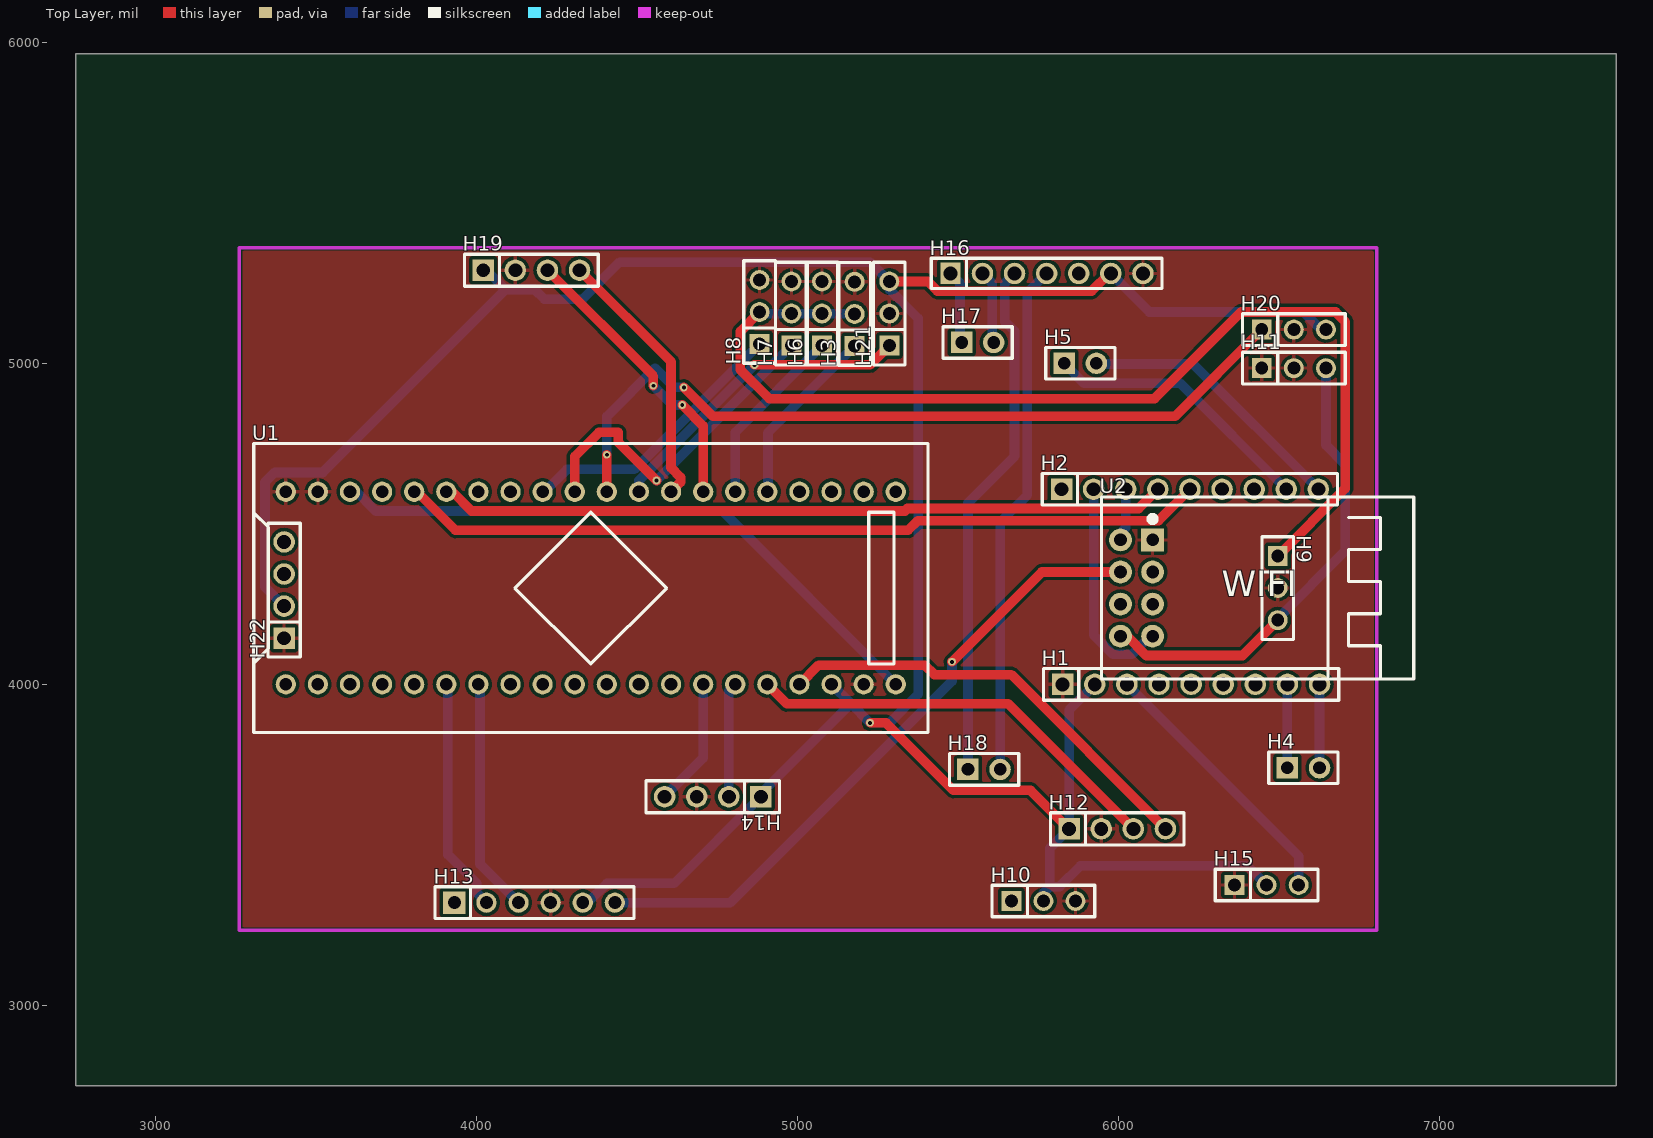
[diagram p0: Top Layer view]
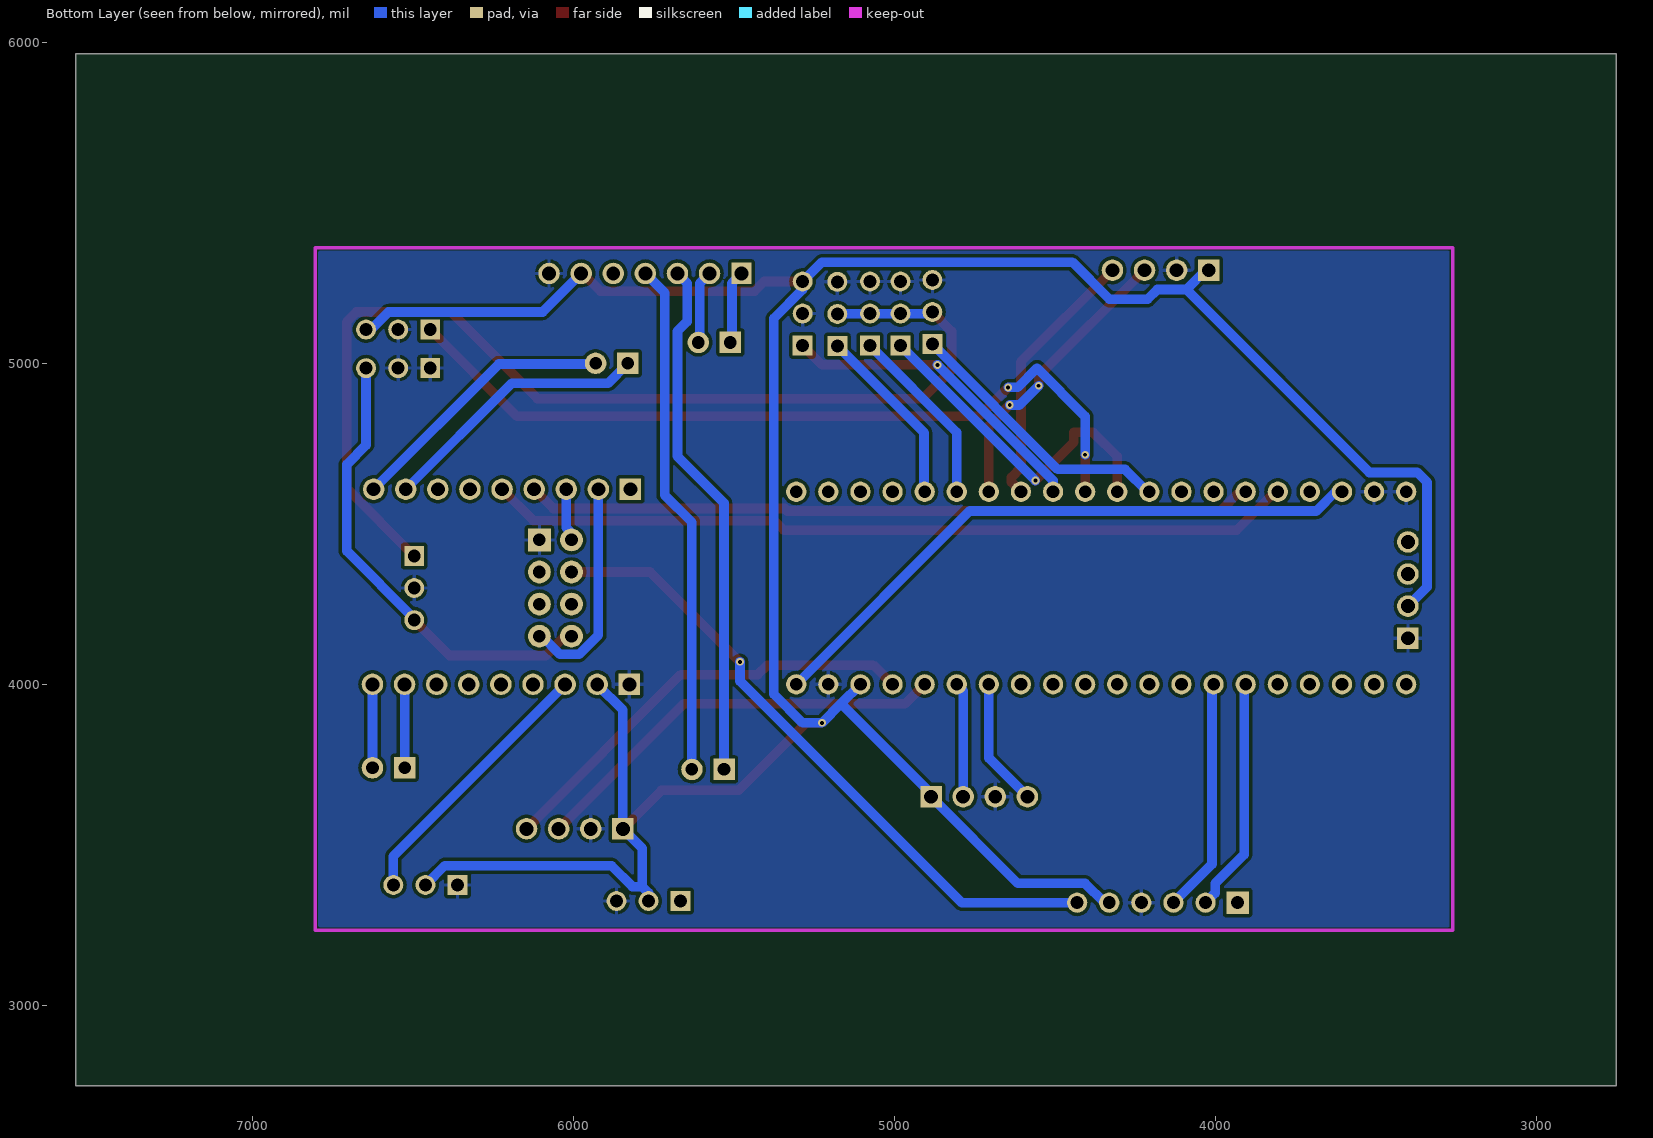
[diagram p1: Bottom Layer view, seen from below]
# Altium PCB MISC51489.pcbdoc
Units mil, origin at the board's own origin, x right, y up, seen from the top; angles counter-clockwise.
Board outline 4800 x 3215 mil, 2 copper layers (Top Layer, Bottom Layer), stack 62.206 mil thick; 24 components, 66 nets, 133 pads, 8 vias.

## Layer stack, top to bottom
Top Solder Mask Layer: solder mask 0.394, Dk 3.3
Top Layer: signal copper 1.379
Dielectric1: surface 59.449, FR4, Dk 4.5
Bottom Layer: signal copper 1.378
Bottom Solder Mask Layer: solder mask 0.394, Dk 3.3

## Board outline
7550,2750 2750,2750 2750,5965 7550,5965

## Design rules (kind name [scope] priority, off if disabled: settings)
BoardOutlineClearance copperThickness2oz_1 [All] p2 off: genericclearance=7.99 ignorepadtopadclearanceinfootprint=FALSE except(0: Arc-SplitContinuation Track-SplitContinuation SMDPad-SplitContinuation THPad-SplitContinuation Via-SplitContinuation Fill-SplitContinuation Region-SplitContinuation Poly-SplitContinuation Text-SplitContinuation Hole-SplitContinuation; 5.98: Arc-CutoutEdge Track-CutoutEdge SMDPad-CutoutEdge THPad-CutoutEdge Via-CutoutEdge Text-CutoutEdge; 6.9: Hole-OutlineEdge Hole-CutoutEdge; 10: Poly-OutlineEdge Poly-CutoutEdge; 11.81: Arc-OutlineEdge Track-OutlineEdge SMDPad-OutlineEdge THPad-OutlineEdge Via-OutlineEdge Fill-OutlineEdge Region-OutlineEdge Text-OutlineEdge Fill-CutoutEdge Region-CutoutEdge)
BoardOutlineClearance Plane_innerPlane_1 [All] p4 off: genericclearance=4.02 ignorepadtopadclearanceinfootprint=FALSE except(0: Arc-SplitContinuation Track-SplitContinuation SMDPad-SplitContinuation THPad-SplitContinuation Via-SplitContinuation Fill-SplitContinuation Region-SplitContinuation Poly-SplitContinuation Text-SplitContinuation Hole-SplitContinuation; 5.98: Arc-CutoutEdge Track-CutoutEdge SMDPad-CutoutEdge THPad-CutoutEdge Via-CutoutEdge Text-CutoutEdge; 6.9: Hole-OutlineEdge Hole-CutoutEdge; 10: Poly-OutlineEdge Poly-CutoutEdge; 11.81: Arc-OutlineEdge Track-OutlineEdge SMDPad-OutlineEdge THPad-OutlineEdge Via-OutlineEdge Fill-OutlineEdge Region-OutlineEdge Text-OutlineEdge Fill-CutoutEdge Region-CutoutEdge)
BoardOutlineClearance Copper_copperRegion_1 [All] p6 off: genericclearance=4.02 ignorepadtopadclearanceinfootprint=FALSE except(0: Arc-SplitContinuation Track-SplitContinuation SMDPad-SplitContinuation THPad-SplitContinuation Via-SplitContinuation Fill-SplitContinuation Region-SplitContinuation Poly-SplitContinuation Text-SplitContinuation Hole-SplitContinuation; 5.98: Arc-CutoutEdge Track-CutoutEdge SMDPad-CutoutEdge THPad-CutoutEdge Via-CutoutEdge Text-CutoutEdge; 6.9: Hole-OutlineEdge Hole-CutoutEdge; 10: Poly-OutlineEdge Poly-CutoutEdge; 11.81: Arc-OutlineEdge Track-OutlineEdge SMDPad-OutlineEdge THPad-OutlineEdge Via-OutlineEdge Fill-OutlineEdge Region-OutlineEdge Text-OutlineEdge Fill-CutoutEdge Region-CutoutEdge)
BoardOutlineClearance copperThickness1oz_1 [All] p8: genericclearance=4.02 ignorepadtopadclearanceinfootprint=FALSE except(0: Arc-SplitContinuation Track-SplitContinuation SMDPad-SplitContinuation THPad-SplitContinuation Via-SplitContinuation Fill-SplitContinuation Region-SplitContinuation Poly-SplitContinuation Text-SplitContinuation Hole-SplitContinuation; 5.98: Arc-CutoutEdge Track-CutoutEdge SMDPad-CutoutEdge THPad-CutoutEdge Via-CutoutEdge Text-CutoutEdge; 6.9: Hole-OutlineEdge Hole-CutoutEdge; 10: Poly-OutlineEdge Poly-CutoutEdge; 11.81: Arc-OutlineEdge Track-OutlineEdge SMDPad-OutlineEdge THPad-OutlineEdge Via-OutlineEdge Fill-OutlineEdge Region-OutlineEdge Text-OutlineEdge Fill-CutoutEdge Region-CutoutEdge)
Clearance copperThickness2oz [All] p1 off: gap=7.99 ignorepadtopadclearanceinfootprint=FALSE except(5.98: SMDPad-Track SMDPad-SMDPad THPad-Track SMDPad-THPad THPad-THPad Track-Via SMDPad-Via THPad-Via Via-Via Fill-SMDPad Region-SMDPad Fill-THPad Region-THPad Fill-Via Region-Via Fill-Fill Fill-Region Region-Region Arc-Track Arc-SMDPad Arc-THPad Arc-Via Fill-Arc Region-Arc Arc-Arc Text-Track SMDPad-Text Text-THPad Text-Via Fill-Text Region-Text Arc-Text Text-Text; 6.9: Hole-Track Hole-SMDPad Hole-THPad Hole-Via Fill-Hole Region-Hole Hole-Arc Hole-Text; 10: Poly-Track Poly-SMDPad Poly-THPad Poly-Via Poly-Fill Poly-Region Poly-Poly Poly-Arc Poly-Text Poly-Hole; 11.81: Fill-Track Region-Track)
Clearance Plane_innerPlane [All] p3 off: gap=4.02 ignorepadtopadclearanceinfootprint=FALSE except(5.98: SMDPad-Track SMDPad-SMDPad THPad-Track SMDPad-THPad THPad-THPad Track-Via SMDPad-Via THPad-Via Via-Via Fill-SMDPad Region-SMDPad Fill-THPad Region-THPad Fill-Via Region-Via Fill-Fill Fill-Region Region-Region Arc-Track Arc-SMDPad Arc-THPad Arc-Via Fill-Arc Region-Arc Arc-Arc Text-Track SMDPad-Text Text-THPad Text-Via Fill-Text Region-Text Arc-Text Text-Text; 6.9: Hole-Track Hole-SMDPad Hole-THPad Hole-Via Fill-Hole Region-Hole Hole-Arc Hole-Text; 10: Poly-Track Poly-SMDPad Poly-THPad Poly-Via Poly-Fill Poly-Region Poly-Poly Poly-Arc Poly-Text Poly-Hole; 11.81: Fill-Track Region-Track)
Clearance Copper_copperRegion [All] p5 off: gap=4.02 ignorepadtopadclearanceinfootprint=FALSE except(5.98: SMDPad-Track SMDPad-SMDPad THPad-Track SMDPad-THPad THPad-THPad Track-Via SMDPad-Via THPad-Via Via-Via Fill-SMDPad Region-SMDPad Fill-THPad Region-THPad Fill-Via Region-Via Fill-Fill Fill-Region Region-Region Arc-Track Arc-SMDPad Arc-THPad Arc-Via Fill-Arc Region-Arc Arc-Arc Text-Track SMDPad-Text Text-THPad Text-Via Fill-Text Region-Text Arc-Text Text-Text; 6.9: Hole-Track Hole-SMDPad Hole-THPad Hole-Via Fill-Hole Region-Hole Hole-Arc Hole-Text; 10: Poly-Track Poly-SMDPad Poly-THPad Poly-Via Poly-Fill Poly-Region Poly-Poly Poly-Arc Poly-Text Poly-Hole; 11.81: Fill-Track Region-Track)
Clearance copperThickness1oz [All] p7: gap=4.02 ignorepadtopadclearanceinfootprint=FALSE except(5.98: SMDPad-Track SMDPad-SMDPad THPad-Track SMDPad-THPad THPad-THPad Track-Via SMDPad-Via THPad-Via Via-Via Fill-SMDPad Region-SMDPad Fill-THPad Region-THPad Fill-Via Region-Via Fill-Fill Fill-Region Region-Region Arc-Track Arc-SMDPad Arc-THPad Arc-Via Fill-Arc Region-Arc Arc-Arc Text-Track SMDPad-Text Text-THPad Text-Via Fill-Text Region-Text Arc-Text Text-Text; 6.9: Hole-Track Hole-SMDPad Hole-THPad Hole-Via Fill-Hole Region-Hole Hole-Arc Hole-Text; 10: Poly-Track Poly-SMDPad Poly-THPad Poly-Via Poly-Fill Poly-Region Poly-Poly Poly-Arc Poly-Text Poly-Hole; 11.81: Fill-Track Region-Track)
DiffPairsRouting differentialPair [All] p1: maxlimit=6 minlimit=6 mostfreqgap=6 toplayer_minwidth=5 toplayer_prefwidth=10 toplayer_maxwidth=100 toplayer_mingap=6 toplayer_prefgap=6 toplayer_maxgap=6 bottomlayer_minwidth=5 bottomlayer_prefwidth=10 bottomlayer_maxwidth=100 bottomlayer_mingap=6 bottomlayer_prefgap=6 bottomlayer_maxgap=6 maxuncoupledlength=10
HoleToHoleClearance otherClearance [All] p1: gap=11.81 allowstackedmicrovias=TRUE
Length netLength [All] p1: minlimit=0 maxlimit=0
MatchedLengths netLengthTolerance [All] p1: tolerance=1000
PasteMaskExpansion pasteMaskExpansion [All] p1: expansion=0
PlaneConnect innerPlane [All] p1: planeconnectstyle=Relief reliefexpansion=20 reliefentries=4 reliefconductorwidth=10 reliefairgap=10
PolygonConnect copperRegion [All] p1: connectstyle=Relief reliefconductorwidth=10 reliefentries=4 polygonreliefangle="90 Angle" airgapwidth=10 via.connectstyle=Relief via.reliefconductorwidth=10 via.reliefentries=4 via.polygonreliefangle="90 Angle" via.airgapwidth=10
RoutingVias viaSize [All] p1: holewidth=12.01 width=24.02 viastyle="Through Hole" minholewidth=11.81 minwidth=19.68 maxholewidth=248.03 maxwidth=393.7
SolderMaskExpansion solderMaskExpansion [IsVia] p1: expansion=-1000 istentingtop=TRUE
SolderMaskExpansion solderMaskExpansion [All] p2: expansion=2 istentingtop=FALSE
Width copperThickness2oz_2 [All] p1 off: maxlimit=100 minlimit=8 preferedwidth=10
Width copperThickness1oz_2 [All] p2: maxlimit=10 minlimit=10 preferedwidth=10 toplayer_minwidth=5 toplayer_maxwidth=100 toplayer_prefwidth=30 bottomlayer_minwidth=5 bottomlayer_maxwidth=100 bottomlayer_prefwidth=30

## Components (designator, comment, footprint, x,y, rotation, side; value= is the part's Value field where it differs from the comment)
H1 "" HDR-TH_9P-P2.54-V-F-1 6225,4000 r0 top
H2 "" HDR-TH_9P-P2.54-V-F-1 6221.35,4607.72 r0 top
H3 "" HDR-TH_3P-P2.54-V-F 5176.94,5153.94 r90 top
H4 "" HDR-TH_2P-P2.54-V-F 6575,3740 r0 top
H5 "" HDR-TH_2P-P2.54-V-F 5880,5000 r0 top
H6 "" HDR-TH_3P-P2.54-V-F 5075,5155 r90 top
H7 "" HDR-TH_3P-P2.54-V-F 4980,5155 r90 top
H8 "" HDR-TH_3P-P2.54-V-F 4880.94,5159.77 r90 top
H9 "" HDR-TH_3P-P2.54-V-F 6495,4300 r270 top
H10 "" HDR-TH_3P-P2.54-V-F 5765,3325 r0 top
H11 "" HDR-TH_3P-P2.54-V-F 6545,4985 r0 top
H12 "" HDR-TH_4P-P2.54-V-F 5995,3550 r0 top
H13 "" HDR-TH_6P-P2.54-V-F 4180,3320 r0 top
H14 "" HDR-TH_4P-P2.54-V-F 4735,3650 r180 top
H15 "" HDR-TH_3P-P2.54-V-F 6460,3375 r0 top
H16 "" HDR-TH_7P-P2.54-V-F 5775,5280 r0 top
H17 "" HDR-TH_2P-P2.54-V-F 5560,5065 r0 top
H18 "" HDR-TH_2P-P2.54-V-F 5580,3735 r0 top
H19 "" HDR-TH_4P-P2.54-V-F 4170,5290 r0 top
H20 "" HDR-TH_3P-P2.54-V-F 6545,5105 r0 top
H21 "" HDR-TH_3P-P2.54-V-F 5285,5155 r90 top
H22 "" HDR-TH_4P-P2.54-V-F 3399.74,4293.7 r90 top
U1 "STM32F103C8T6-Card" CONN-TH_L53.3-W22.9_STM32F103C8T6-CARD 4355,4300 r0 top
U2 "Ai-Thinker ESP-01S ESP8266" WIFIM-TH_8P-L24.7-W14.4-P2.54 6055,4300 r0 top

## Footprints (in the part's own frame and the unit in brackets; to place one, negate y for a bottom-side part, rotate by r counter-clockwise, add the part's x,y. Pads: shape width x height; smd on the part's side, far side on the other; paste and mask are expansions set on the pad)
CONN-TH_L53.3-W22.9_STM32F103C8T6-CARD [mm]
  round 1.6 hole 1: 1(-24.13,-7.62) 2(-21.59,-7.62) 3(-19.05,-7.62) 4(-16.51,-7.62) 5(-13.97,-7.62) 6(-11.43,-7.62) 7(-8.89,-7.62) 8(-6.35,-7.62) 9(-3.81,-7.62) 10(-1.27,-7.62) 11(1.27,-7.62) 12(3.81,-7.62) 13(6.35,-7.62) 14(8.89,-7.62) 15(11.43,-7.62) 16(13.97,-7.62) 17(16.51,-7.62) 18(19.05,-7.62) 19(21.59,-7.62) 20(24.13,-7.62) 21(24.13,7.62) 22(21.59,7.62) 23(19.05,7.62) 24(16.51,7.62) 25(13.97,7.62) 26(11.43,7.62) 27(8.89,7.62) 28(6.35,7.62) 29(3.81,7.62) 30(1.27,7.62) 31(-1.27,7.62) 32(-3.81,7.62) 33(-6.35,7.62) 34(-8.89,7.62) 35(-11.43,7.62) 36(-13.97,7.62) 37(-16.51,7.62) 38(-19.05,7.62) 39(-21.59,7.62) 40(-24.13,7.62)
  silkscreen extent -26.67,-11.43 26.67,11.43
HDR-TH_2P-P2.54-V-F [mm]
  rect 1.7x1.7 hole 1: 1(-1.27,0)
  round 1.7 hole 1: 2(1.27,0)
  silkscreen extent -2.74,-1.25 2.74,1.25
HDR-TH_3P-P2.54-V-F [mil]
  rect 62x62 hole 40.16: 1(-100,0)
  round 62 hole 40.16: 2(0,0) 3(100,0)
  silkscreen extent -160,-49 160,49
HDR-TH_4P-P2.54-V-F [mm]
  rect 1.7x1.7 hole 1.1: 1(-3.81,0)
  round 1.7 hole 1.1: 2(-1.27,0) 3(1.27,0) 4(3.81,0)
  silkscreen extent -5.29,-1.27 5.29,1.27
HDR-TH_6P-P2.54-V-F [mm]
  rect 1.8x1.8 hole 1.02: 1(-6.35,0)
  round 1.6 hole 1.02: 2(-3.81,0) 3(-1.27,0) 4(1.27,0) 5(3.81,0) 6(6.35,0)
  silkscreen extent -7.87,-1.25 7.87,1.25
HDR-TH_7P-P2.54-V-F [mm]
  rect 1.575x1.7 hole 1.1: 1(-7.62,0)
  round 1.7 hole 1.1: 2(-5.08,0) 3(-2.54,0) 4(0,0) 5(2.54,0) 6(5.08,0) 7(7.62,0)
  silkscreen extent -9.13,-1.2 9.13,1.2
HDR-TH_9P-P2.54-V-F-1 [mm]
  rect 1.7x1.7 hole 1.1: 1(-10.16,0)
  round 1.7 hole 1.1: 2(-7.62,0) 3(-5.08,0) 4(-2.54,0) 5(0,0) 6(2.54,0) 7(5.08,0) 8(7.62,0) 9(10.16,0)
  silkscreen extent -11.68,-1.25 11.68,1.25
WIFIM-TH_8P-L24.7-W14.4-P2.54 [mm]
  rect 1.8x1.8 hole 1 paste+0 mask+0.05: 1(1.27,3.81)
  round 1.8 hole 1 paste+0 mask+0.05: 2(1.27,1.27) 3(1.27,-1.27) 4(1.27,-3.81) 5(-1.27,3.81) 6(-1.27,1.27) 7(-1.27,-1.27) 8(-1.27,-3.81)
  silkscreen extent -2.77,-7.19 21.93,7.24

## Via types
v1: diameter 24.02, hole 12, Top Layer to Bottom Layer, 8 vias

## Nets (pads, with @x,y where several pads share a name; then routed paths per layer and width w, separated by ;. In a path a pad name is that pad's centre, name@x,y a point inside that pad or via, vN(x,y) a via of type N, cw(c..) or ccw(c..) an arc to the next point about the centre after c; other vN are vias at no path point)
3.3V: U1.20 U1.38 | length 1948.5
  Bottom Layer w30: U1.38 3625.01,4600 3685.01,4540 4765,4540 U1.20
3V3: H2.1
$1N17145: H1.9 H4.2 | length 260
  Bottom Layer w30: H4.2 H1.9
$1N17146: H1.8 H4.1 | length 260
  Bottom Layer w30: H4.1 H1.8
$1N17147: H2.9 H5.2 | length 854.2
  Bottom Layer w30: H5.2 5931.35,4997.72 6231.35,4997.72 H2.9
$1N17148: H2.8 H5.1 | length 854.2
  Bottom Layer w30: H5.1 5831.35,4997.72 5891.35,4937.72 6191.35,4937.72 H2.8
$1N17189: H16.1 H17.1 | length 229.5
  Bottom Layer w30: H16.1 5505,5250 5505,5070 H17.1
$1N17190: H16.2 H17.2 | length 229.5
  Bottom Layer w30: H16.2 5605,5250 5605,5070 H17.2
$1N17191: H16.3 H18.1 | length 1629.9
  Bottom Layer w30: H18.1 5530,4565 5675,4710 5675,5100 5645,5130 5645,5250 H16.3
$1N17192: H16.4 H18.2 | length 1605.1
  Bottom Layer w30: H18.2 5630,4505 5715,4590 5715,5220 H16.4
+5V: H1.2 H10.2 H12.1 H13.5 H14.1 H15.2 H16.6 H19.1 H20.3 H21.3 H22.2 U1.18 | length 9253.7
  Top Layer w30: v1(5225,3880) 5275,3880 5485,3670 5725,3670 H12.1 ; H21.3 5405,5255 5435,5225 5915,5225 5970,5280 H16.6
  Bottom Layer w30: H22.2 3340,4303.44 3340,4630 3370,4660 3520,4660 4090,5230 ; H19.1 4030,5290 4090,5230 ; H13.5 4345,3320 4405,3380 4615,3380 H14.1 4885,3660 5165,3940 ; U1.18 5165,3940 ; H10.2 5765,3350 5785,3370 ; H1.2 5845,3920 H12.1 5785,3490 5785,3370 ; H16.6 6095,5160 6575,5160 6630,5105 H20.3 ; H15.2 6400,3435 5880,3435 5815,3370 5785,3370 ; 4090,5230 4180,5230 4210,5200 4330,5200 4445,5315 5225,5315 H21.3 5285,5230 5375,5140 5375,3970 5285,3880 v1(5225,3880) 5165,3940
BAT_3.7V: H9.3 H11.3 U2.8 | length 1457.3
  Top Layer w30: U2.8 6025,4150 6085,4090 6385,4090 H9.3
  Bottom Layer w30: H9.3 6495,4205 6705,4415 6705,4685 6645,4745 H11.3
EN: H13.6 U2.6 | length 2036.8
  Top Layer w30: v1(5480,4070) 5760,4350 U2.6
  Bottom Layer w30: H13.6 4790,3320 5480,4010 v1(5480,4070)
GND: H1.1 H3.3 H6.3 H7.3 H8.3 H9.2 H10.3 H11.1 H11.2 H12.2 H13.4 H14.3 H15.1 H16.7 H19.2 H20.2 H21.2 H22.1 U1.19 U1.39 U1.40 U2.1
IO0: U2.3
IO2: U2.2
MOTOR_+5V: H3.2 H6.2 H7.2 H8.2 H9.1 | length 3365.2
  Top Layer w30: H8.2 4820.94,5099.77 4820.94,4979.77 4910.94,4889.77 6110.94,4889.77 6380.94,5159.77 6675,5159.77 6705,5129.77 6705,4610 H9.1
  Bottom Layer w30: H8.2 4885.23,5159.77 4890,5155 H7.2 H6.2 5086.94,5153.94 H3.2
MUTE: H1.7
NRST: U1.37
PA0: H3.1 U1.25 | length 566.2
  Bottom Layer w30: U1.25 4906.94,4603.94 4906.94,4783.94 H3.1
PA0/: H2.7
PA1: H6.1 U1.26 | length 566.8
  Bottom Layer w30: U1.26 4805,4785 H6.1
PA1/: H2.6
PA2: H19.3 U1.27 | length 908.5
  Top Layer w30: H19.3 4550,4960 v1(4550,4930) ; v1(4640,4870) 4705,4805 U1.27
  Bottom Layer w30: v1(4550,4930) 4610,4870 v1(4640,4870)
PA3: H19.4 U1.28 | length 832.9
  Top Layer w30: H19.4 4605,5004.99 4605,4675 4635,4645 4635,4630 U1.28
PA4: H21.1 U1.29 | length 989
  Top Layer w30: v1(4865,4995) 5225,4995 H21.1
  Bottom Layer w30: U1.29 4505,4635 v1(4865,4995)
PA4/: H1.6
PA5: H20.1 U1.30 | length 2511.1
  Top Layer w30: U1.30 v1(4405,4715) ; v1(4645,4925) 4735,4835 6175,4835 H20.1
  Bottom Layer w30: v1(4405,4715) 4405,4835 4555,4985 4615,4925 v1(4645,4925)
PA5/: H2.3 U2.5 | length 164.5
  Bottom Layer w30: U2.5 6005,4471.37 6021.35,4487.72 H2.3
PA6: H7.1 U1.31 | length 1069.7
  Top Layer w30: U1.31 4305,4710 4380,4785 4440,4785 4440,4755 v1(4560,4635)
  Bottom Layer w30: v1(4560,4635) H7.1
PA6/: H2.2 U2.4 | length 685.9
  Bottom Layer w30: H2.2 5921.35,4153.65 5981.35,4093.65 6041.35,4093.65 6097.7,4150 U2.4
PA7: H8.1 U1.32 | length 866.4
  Bottom Layer w30: U1.32 4211.17,4600 4280.94,4669.77 4490.94,4669.77 H8.1
PA8: U1.5
PA9: H13.2 U1.6 | length 731.8
  Bottom Layer w30: U1.6 3910,3995 3910,3470 4000,3380 4000,3350 H13.2
PA10: H13.3 U1.7 | length 731.8
  Bottom Layer w30: U1.7 4010,3995 4010,3440 H13.3
PA11: U1.8
PA12: U1.9
PA15: U1.10
PB0: U1.33
PB1: U1.34
PB3: U1.11
PB4: U1.12
PB5: U1.13
PB5/: H1.3 H15.3 | length 846.6
  Bottom Layer w30: H1.3 6560,3465 H15.3
PB6: H14.4 U1.14 | length 399.7
  Bottom Layer w30: H14.4 4705,3770 U1.14
PB6/: H1.4
PB7: H14.2 U1.15 | length 358.3
  Bottom Layer w30: H14.2 4785,3980 U1.15
PB8: H12.3 U1.16 | length 1326.4
  Top Layer w30: U1.16 4965,3940 5655,3940 H12.3
PB9: H12.4 U1.17 | length 1376.1
  Top Layer w30: U1.17 5065,4060 5395,4060 5425,4030 5665,4030 H12.4
PB10: H2.4 U1.35 | length 2269.3
  Top Layer w30: U1.35 3923.64,4600 3983.64,4540 5333.63,4540 5341.35,4547.72 6061.35,4547.72 H2.4
PB11: H2.5 U1.36 | length 2519
  Top Layer w30: U1.36 3813.64,4600 3933.64,4480 5343.63,4480 5373.63,4510 6123.63,4510 H2.5
PB12: U1.1
PB13: U1.2
PB14: U1.3
PB15: U1.4
PC4/: H1.5
PC13: U1.22
PC14: U1.23
PC15: U1.24
RST: U2.7
SCK: H22.3
SDA: H22.4
STATE: H13.1
TYPE-C_+5V: H10.1
VBAT: H16.5
VBT: U1.21

## Polygon pours and split planes (outlines as drawn)
GND on Top Layer (solid, remove dead copper, pour order 0): 3000,5615 3000,3000 7300,3000 7300,5615
GND on Bottom Layer (solid, remove dead copper, pour order 2): 3110,5715 3110,3040 7110,3040 7110,5715

## Keep-outs
Board Outline Layer:
  lines w10: 3260,3234.02 3260,5360 6803.31,5360 6803.31,3234.02 3260,3234.02